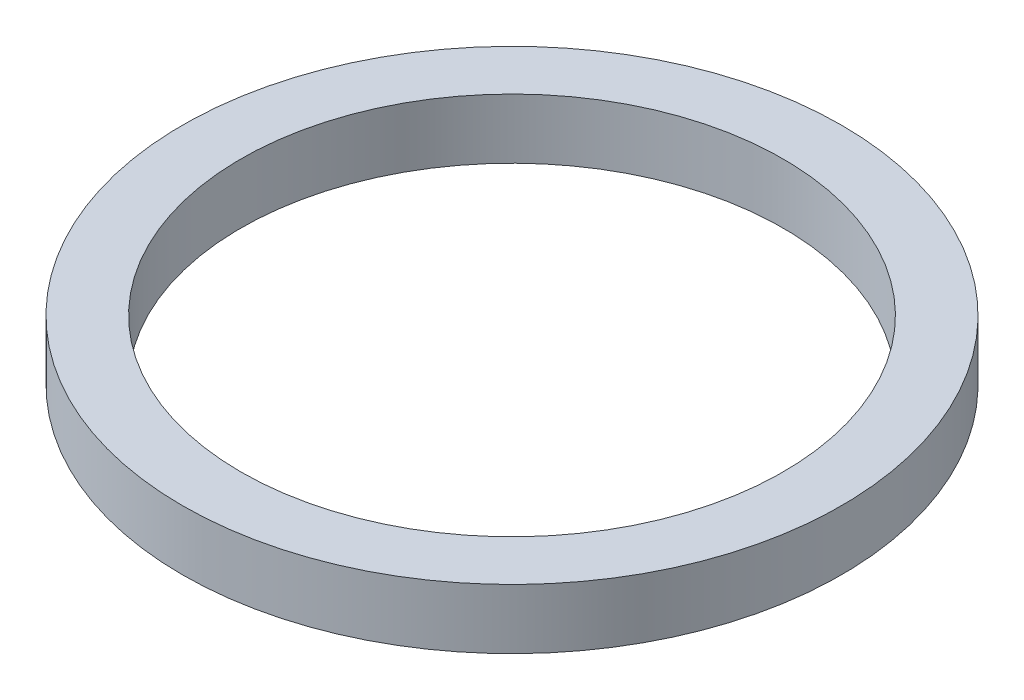
from build123d import *

# Parameters (mm, degrees)
SKETCH_1_R      = 16.5
SKETCH_1_R_2    = 13.575
EXTRUDE_1_DEPTH = 3


with BuildPart() as part:
    # 草图1 → 凸台-拉伸1 (new body)
    with BuildSketch(Plane(origin=(0, 0, 0), x_dir=(1, 0, 0), z_dir=(0, 1, 0))):
        with Locations(Location((0, 0, 0), (0, 0, 270))):
            Circle(SKETCH_1_R)
        with Locations(Location((0, 0, 0), (0, 0, 270))):
            Circle(SKETCH_1_R_2, mode=Mode.SUBTRACT)
    extrude(amount=EXTRUDE_1_DEPTH)


solid = part.part
